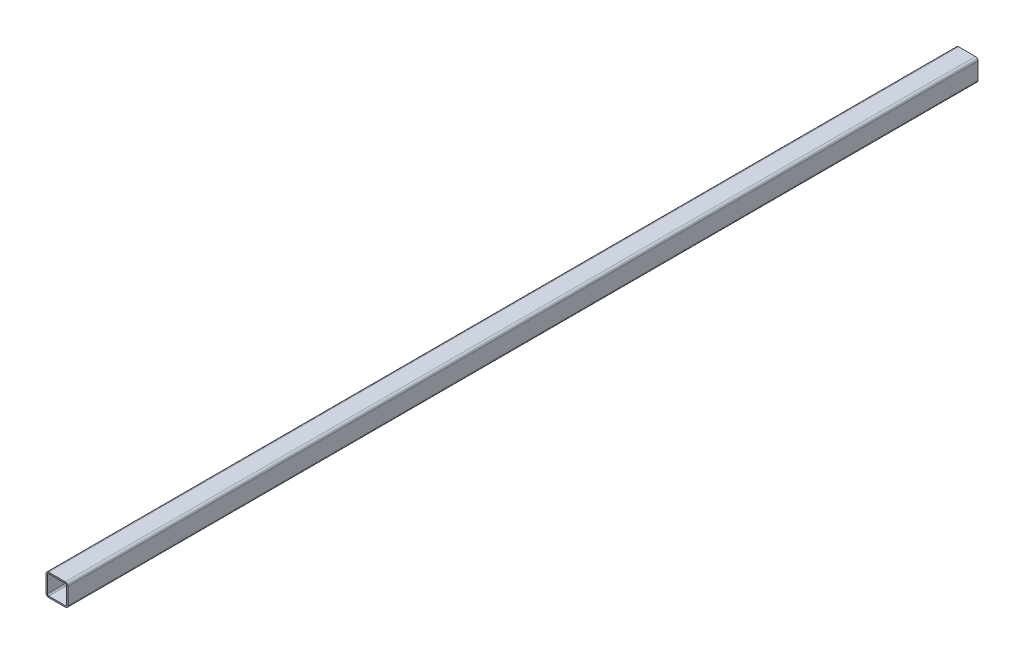
SolidWorks part; units mm, degrees
material "Q235B"
ref_plane "前视基准面" through (0, 0, 0) normal (0, 0, 1) x (1, 0, 0)
ref_plane "上视基准面" through (0, 0, 0) normal (0, 1, 0) x (1, 0, 0)
ref_plane "右视基准面" through (0, 0, 0) normal (1, 0, 0) x (0, 0, -1)
other "Configuration Table"
sketch "草图1" plane through (0, 0, 0) normal (1, 0, 0) x (0, 0, -1)
  line L0 (-1035, 0) -> (1035, 0)
other "Gb／6728-1986方形空心型钢 050 X 50 X 3(1)"
ref_plane "基准面1" through (0, 0, 1035) normal (0, 0, -1) x (0, 1, 0)
sketch "Sketch1" plane through (0, 0, 1035) normal (0, 0, -1) x (0, 1, 0)
  line L0 (-19, -22) -> (19, -22)
  line L1 (-22, -19) -> (-22, 19)
  line L2 (19, 22) -> (-19, 22)
  line L3 (22, 19) -> (22, -19)
  line L4 (-19, -25) -> (19, -25)
  line L5 (-25, -19) -> (-25, 19)
  line L6 (19, 25) -> (-19, 25)
  line L7 (25, 19) -> (25, -19)
  arc A0 (25, 19) -> (19, 25) centre (19, 19) ccw
  arc A1 (19, -25) -> (25, -19) centre (19, -19) ccw
  arc A2 (-25, -19) -> (-19, -25) centre (-19, -19) ccw
  arc A3 (-19, 25) -> (-25, 19) centre (-19, 19) ccw
  arc A4 (-19, 22) -> (-22, 19) centre (-19, 19) ccw
  arc A5 (22, 19) -> (19, 22) centre (19, 19) ccw
  arc A6 (19, -22) -> (22, -19) centre (19, -19) ccw
  arc A7 (-22, -19) -> (-19, -22) centre (-19, -19) ccw
  point P0 (-25, 0)
  point P1 (25, 0)
  point P2 (0, 25)
  point P3 (0, -25)
  point P4 (0, 0)
  point P5 (-25, -25)
  point P6 (25, -25)
  point P7 (25, 25)
  point P8 (-25, 25)
  point P33 (0, 0)
  dimension "D1" = 6
  dimension "Thickness" = 3
  dimension "V_leg" = 50
equation "\"D2@草图1\"=\"D1@草图1\"/2"
